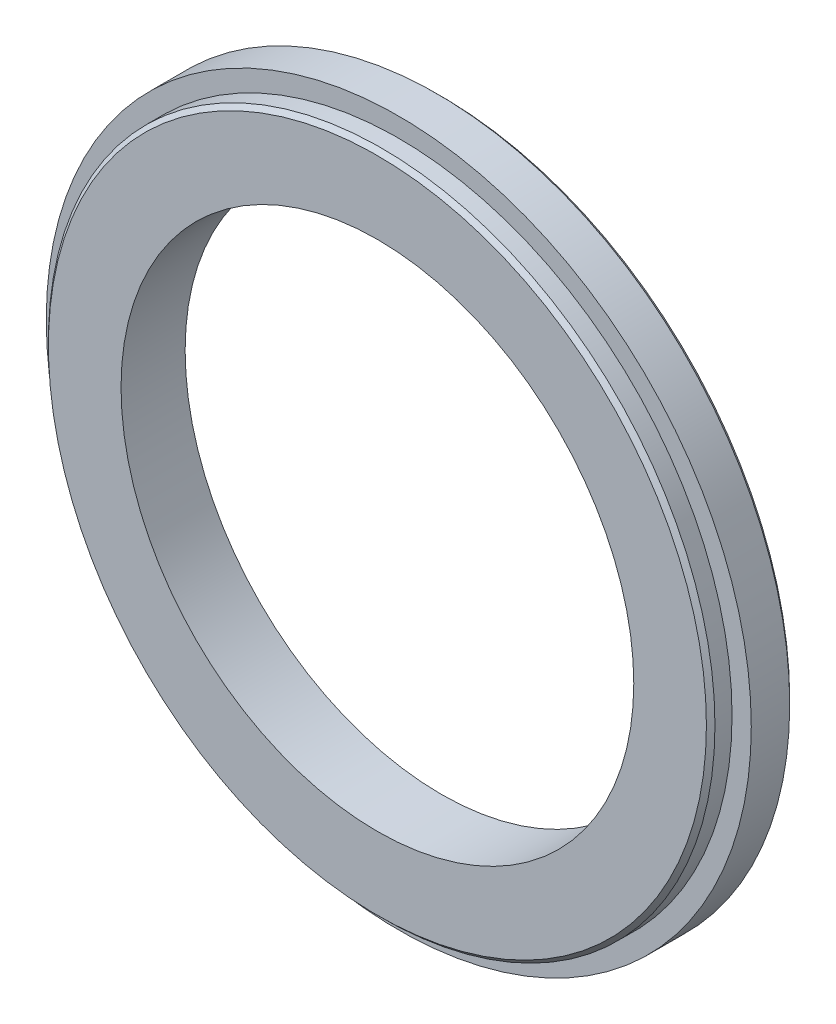
from build123d import *

# Parameters (mm, degrees)
SKETCH1_R             = 82.5
SKETCH1_R_2           = 60
BOSS_EXTRUDE1_DEPTH   = 10
SKETCH2_R             = 78
SKETCH2_R_2           = 60
BOSS_EXTRUDE2_DEPTH   = 5
CHAMFER1_SIZE         = 1
M8_TAPPED_HOLE1_D     = 6.8
M8_TAPPED_HOLE1_DEPTH = 12
M8_TAPPED_HOLE1_TIP   = 2.042926105


with BuildPart() as part:
    # Sketch1 → Boss-Extrude1 (new body)
    with BuildSketch(Plane.XY):
        Circle(SKETCH1_R)
        Circle(SKETCH1_R_2, mode=Mode.SUBTRACT)
    extrude(amount=BOSS_EXTRUDE1_DEPTH)

    # Sketch2 → Boss-Extrude2 (add)
    with BuildSketch(Plane.XY.offset(10)):
        Circle(SKETCH2_R)
        Circle(SKETCH2_R_2, mode=Mode.SUBTRACT)
    extrude(amount=BOSS_EXTRUDE2_DEPTH)

    # Chamfer1
    chamfer1_edges = [part.edges().sort_by_distance(p)[0] for p in [
        (-78, 0, 15),
        (-82.5, 0, 0),
    ]]
    chamfer(chamfer1_edges, length=CHAMFER1_SIZE)

    # M8 Tapped Hole1
    with Locations(Plane(origin=(35, 60.621778265, 0), x_dir=(-1, 0, 0), z_dir=(0, 0, -1))):
        with Locations((0, 0), (70, 0), (105, -60.621778265), (70, -121.24355653), (0, -121.24355653), (-35, -60.621778265)):
            Hole(M8_TAPPED_HOLE1_D / 2, depth=M8_TAPPED_HOLE1_DEPTH)
            with Locations((0, 0, -(M8_TAPPED_HOLE1_DEPTH + M8_TAPPED_HOLE1_TIP / 2))):  # 118° drill point
                Cone(0, M8_TAPPED_HOLE1_D / 2, M8_TAPPED_HOLE1_TIP, mode=Mode.SUBTRACT)


solid = part.part
